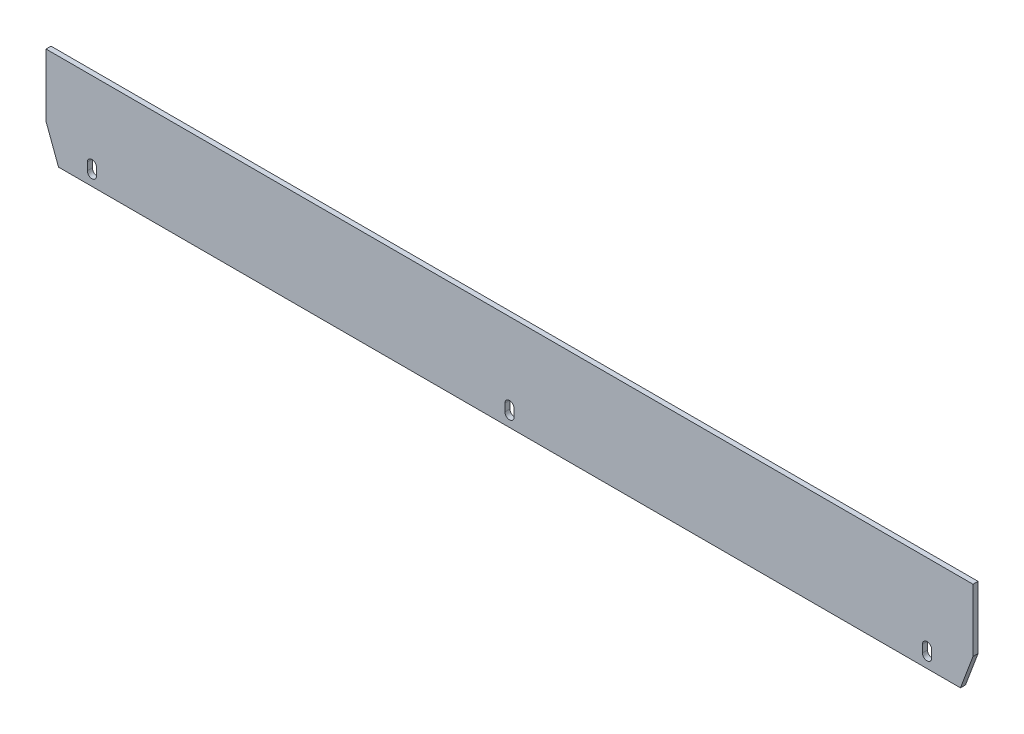
from build123d import *

# Parameters (mm, degrees)
SKETCH1_W           = 1110
SKETCH1_H           = 115
BOSS_EXTRUDE1_DEPTH = 6
CUT_EXTRUDE1_DEPTH  = 6


with BuildPart() as part:
    # Sketch1 → Boss-Extrude1 (new body)
    with BuildSketch(Plane.XY):
        Rectangle(SKETCH1_W, SKETCH1_H)
    extrude(amount=BOSS_EXTRUDE1_DEPTH)

    # Sketch2 → Cut-Extrude1 (cut)
    with BuildSketch(Plane.XY.offset(6)):
        with BuildLine():
            Line((-494.5, -35), (-494.5, -44))
            ThreePointArc((-494.5, -44), (-500, -49.5), (-505.5, -44))
            Line((-505.5, -44), (-505.5, -35))
            ThreePointArc((-505.5, -35), (-500, -29.5), (-494.5, -35))
        make_face()
        with BuildLine():
            Line((5.5, -35), (5.5, -44))
            ThreePointArc((5.5, -44), (0, -49.5), (-5.5, -44))
            Line((-5.5, -44), (-5.5, -35))
            ThreePointArc((-5.5, -35), (0, -29.5), (5.5, -35))
        make_face()
        with BuildLine():
            Line((494.5, -44), (494.5, -35))
            ThreePointArc((494.5, -35), (500, -29.5), (505.5, -35))
            Line((505.5, -35), (505.5, -44))
            ThreePointArc((505.5, -44), (500, -49.5), (494.5, -44))
        make_face()
        Polygon((-555, -17.5), (-540, -57.5), (-555, -57.5), align=None)
        Polygon((555, -17.5), (540, -57.5), (555, -57.5), align=None)
    extrude(amount=-CUT_EXTRUDE1_DEPTH, mode=Mode.SUBTRACT)


solid = part.part
